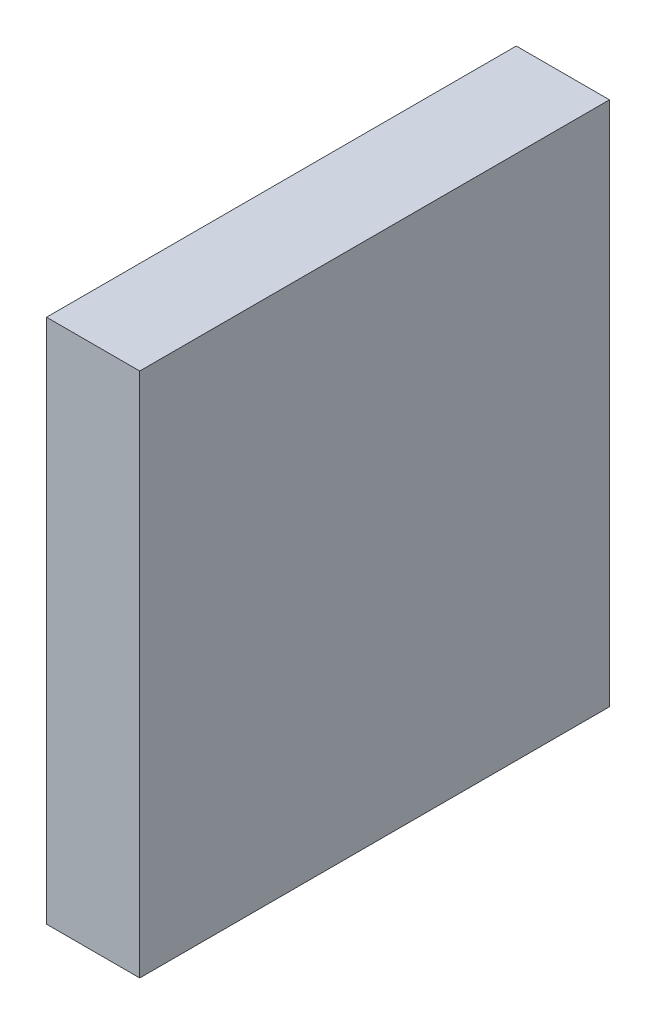
SolidWorks part; units mm, degrees
material "Q345B"
ref_plane "Front Plane" through (0, 0, 0) normal (0, 0, 1) x (1, 0, 0)
ref_plane "Top Plane" through (0, 0, 0) normal (0, 1, 0) x (1, 0, 0)
ref_plane "Right Plane" through (0, 0, 0) normal (1, 0, 0) x (0, 0, -1)
sketch "Sketch2" plane through (0, 0, 0) normal (0, 1, 0) x (1, 0, 0)
  line L0 (-131.395, 0) -> (113.7022, 0) construction
  line L1 (0, 164.1787) -> (0, -121.5078) construction
  line L3 (-12.5, 63) -> (12.5, 63)
  line L4 (-12.5, 63) -> (-12.5, -63)
  line L5 (-12.5, -63) -> (12.5, -63)
  line L6 (12.5, 63) -> (12.5, -63)
  dimension "D1" = 126
  dimension "D2" = 25
  dimension "D3" = 12.5
extrude "Boss-Extrude1" add sketch "Sketch2" along normal mid plane 141
